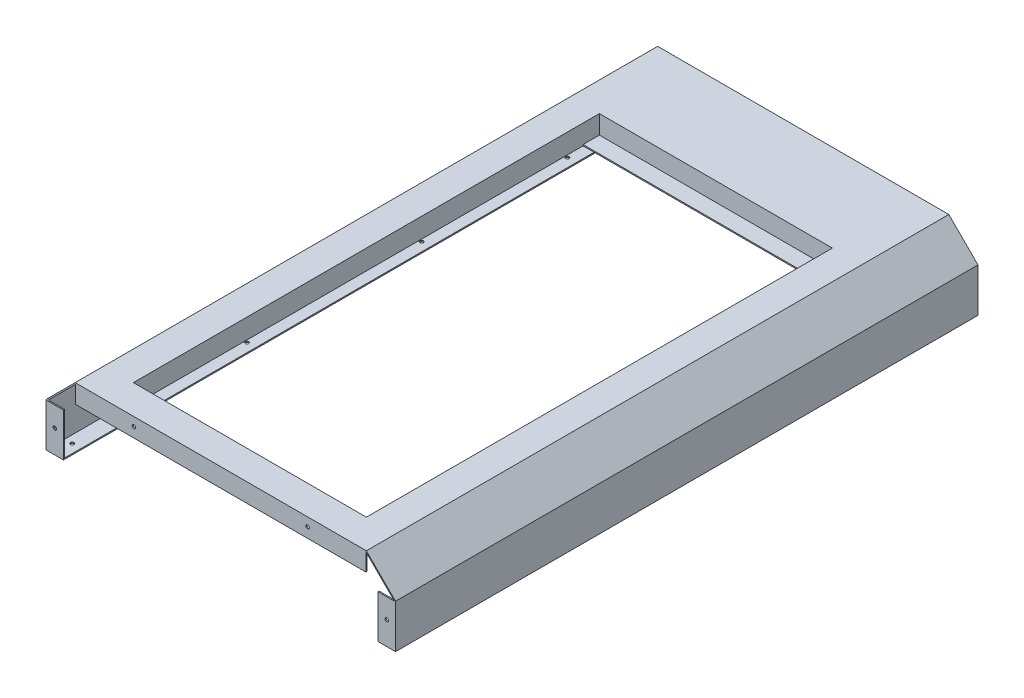
from build123d import *

# Parameters (mm, degrees)
EXTRUDE_1_DEPTH     = 1000
SHELL_1_T           = -2
SKETCH_3_W          = 400
SKETCH_3_H          = 800
CUT_EXTRUDE_1_DEPTH = 30
SKETCH_4_W          = 404
SKETCH_4_H          = 804
SKETCH_4_W_2        = 400
SKETCH_4_H_2        = 800
EXTRUDE_2_DEPTH     = 34
EXTRUDE_3_DEPTH     = 2
SKETCH_6_W          = 600
SKETCH_6_H          = 200
CUT_EXTRUDE_2_DEPTH = 1044
SKETCH_10_W         = 600
SKETCH_10_H         = 425
CUT_EXTRUDE_4_DEPTH = 1005
SKETCH_11_W         = 28
SKETCH_11_H         = 998
EXTRUDE_5_DEPTH     = 2
SKETCH_12_W         = 498.34314575
SKETCH_12_H         = 30
SKETCH_12_W_2       = 28
SKETCH_12_H_2       = 72.171572875
EXTRUDE_6_DEPTH     = 2
SKETCH_13_R         = 3
CUT_EXTRUDE_5_DEPTH = 1280
SKETCH_14_R         = 3
CUT_EXTRUDE_6_DEPTH = 10
SKETCH_15_R         = 3
CUT_EXTRUDE_7_DEPTH = 28
SKETCH_16_R         = 3
CUT_EXTRUDE_8_DEPTH = 10


with BuildPart() as part:
    # 草图1 → 凸台-拉伸1 (new body)
    with BuildSketch(Plane.XY):
        Polygon((0, 700), (50, 750), (550, 750), (600, 700), (600, 0), (0, 0), align=None)
    extrude(amount=EXTRUDE_1_DEPTH)

    # 抽壳1
    shell_1_openings = [part.faces().sort_by_distance(p)[0] for p in [
        (300, 372.998137803, 1000),
    ]]
    offset(amount=SHELL_1_T, openings=shell_1_openings, kind=Kind.INTERSECTION)

    # 草图3 → 切除-拉伸1 (cut)
    with BuildSketch(Plane(origin=(0, 750, 0), x_dir=(1, 0, 0), z_dir=(0, 1, 0))):
        with Locations((300, -550)):
            Rectangle(SKETCH_3_W, SKETCH_3_H)
    extrude(amount=-CUT_EXTRUDE_1_DEPTH, mode=Mode.SUBTRACT)

    # 草图4 → 凸台-拉伸2 (add)
    with BuildSketch(Plane(origin=(0, 750, 0), x_dir=(1, 0, 0), z_dir=(0, 1, 0))):
        with Locations((300, -550)):
            Rectangle(SKETCH_4_W, SKETCH_4_H)
        with Locations((300, -550)):
            Rectangle(SKETCH_4_W_2, SKETCH_4_H_2, mode=Mode.SUBTRACT)
    extrude(amount=-EXTRUDE_2_DEPTH)

    # 草图5 → 凸台-拉伸3 (add)
    with BuildSketch(Plane.XZ.offset(-716)):
        Polygon((128, 178), (472, 178), (472, 922), (128, 922), (100, 922), (100, 950), (500, 950), (500, 150), (100, 150), (100, 178), align=None)
    extrude(amount=-EXTRUDE_3_DEPTH)

    # 草图6 → 切除-拉伸2 (cut)
    with BuildSketch(Plane(origin=(0, 0, 0), x_dir=(-1, 0, 0), z_dir=(0, 0, -1))):
        with Locations((-300, 100)):
            Rectangle(SKETCH_6_W, SKETCH_6_H)
    extrude(amount=-CUT_EXTRUDE_2_DEPTH, mode=Mode.SUBTRACT)

    # 草图10 → 切除-拉伸4 (cut)
    with BuildSketch(Plane(origin=(0, 0, 0), x_dir=(-1, 0, 0), z_dir=(0, 0, -1))):
        with Locations((-300, 412.5)):
            Rectangle(SKETCH_10_W, SKETCH_10_H)
    extrude(amount=-CUT_EXTRUDE_4_DEPTH, mode=Mode.SUBTRACT)

    # 草图11 → 凸台-拉伸5 (add)
    with BuildSketch(Plane.XZ.offset(-625)):
        with Locations((16, 501)):
            Rectangle(SKETCH_11_W, SKETCH_11_H)
        with Locations((584, 501)):
            Rectangle(SKETCH_11_W, SKETCH_11_H)
    extrude(amount=-EXTRUDE_5_DEPTH)

    # 草图12 → 凸台-拉伸6 (add)
    with BuildSketch(Plane.XY.offset(1000)):
        with Locations((300, 733)):
            Rectangle(SKETCH_12_W, SKETCH_12_H)
        with Locations((16, 663.085786438)):
            Rectangle(SKETCH_12_W_2, SKETCH_12_H_2)
        with Locations((584, 663.085786438)):
            Rectangle(SKETCH_12_W_2, SKETCH_12_H_2)
    extrude(amount=-EXTRUDE_6_DEPTH)

    # 草图13 → 切除-拉伸5 (cut)
    with BuildSketch(Plane.XY.offset(1000)):
        with Locations((585, 665)):
            Circle(SKETCH_13_R)
        with Locations((15, 665)):
            Circle(SKETCH_13_R)
    extrude(amount=-CUT_EXTRUDE_5_DEPTH, mode=Mode.SUBTRACT)

    # 草图14 → 切除-拉伸6 (cut)
    with BuildSketch(Plane.XZ.offset(-625)):
        with Locations((15, 970)):
            Circle(SKETCH_14_R)
        with Locations((15, 670)):
            Circle(SKETCH_14_R)
        with Locations(Location((585, 120, 0), (0, 0, 270))):
            Circle(SKETCH_14_R)
        with Locations((15, 370)):
            Circle(SKETCH_14_R)
        with Locations(Location((585, 370, 0), (0, 0, 270))):
            Circle(SKETCH_14_R)
        with Locations((15, 120)):
            Circle(SKETCH_14_R)
        with Locations(Location((585, 670, 0), (0, 0, 270))):
            Circle(SKETCH_14_R)
        with Locations(Location((585, 970, 0), (0, 0, 270))):
            Circle(SKETCH_14_R)
    extrude(amount=-CUT_EXTRUDE_6_DEPTH, mode=Mode.SUBTRACT)

    # 草图15 → 切除-拉伸7 (cut)
    with BuildSketch(Plane.XY.offset(1000)):
        with Locations((150.828427125, 735)):
            Circle(SKETCH_15_R)
        with Locations((449.171572875, 735)):
            Circle(SKETCH_15_R)
    extrude(amount=-CUT_EXTRUDE_7_DEPTH, mode=Mode.SUBTRACT)

    # 草图16 → 切除-拉伸8 (cut)
    with BuildSketch(Plane(origin=(0, 0, 0), x_dir=(-1, 0, 0), z_dir=(0, 0, -1))):
        with Locations((-450, 735)):
            Circle(SKETCH_16_R)
        with Locations((-150, 734.726066428)):
            Circle(SKETCH_16_R)
    extrude(amount=-CUT_EXTRUDE_8_DEPTH, mode=Mode.SUBTRACT)


solid = part.part
